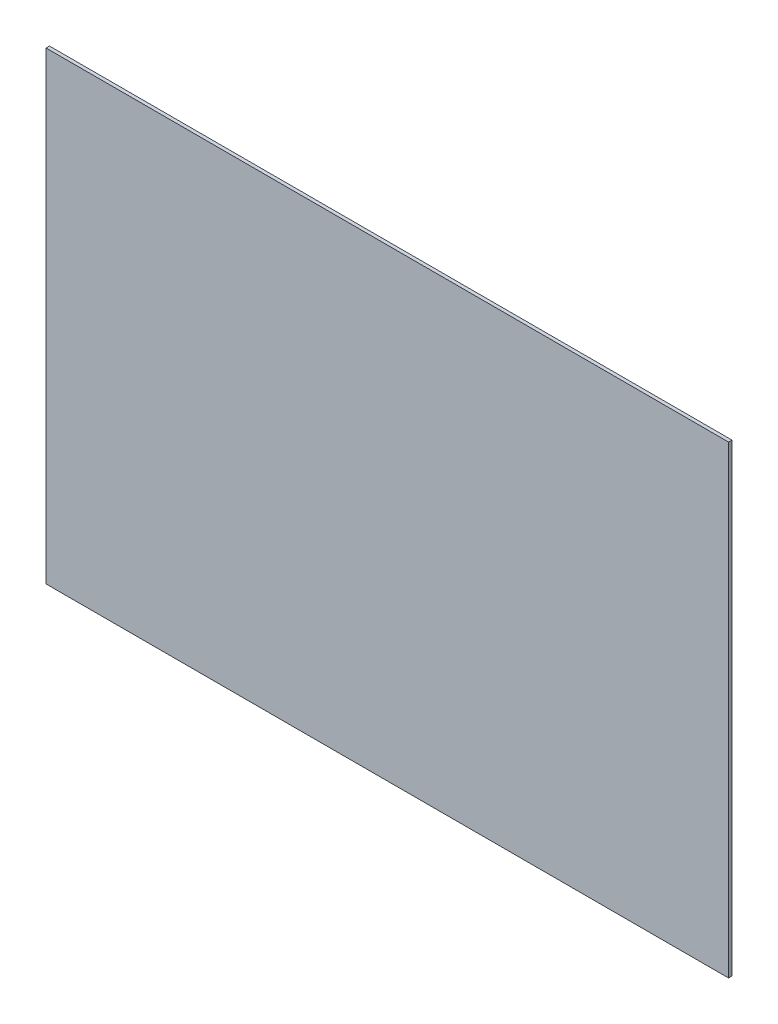
SolidWorks part; units mm, degrees
material "PMMA(有机玻璃)"
ref_plane "前视" through (0, 0, 0) normal (0, 0, 1) x (1, 0, 0)
ref_plane "上视" through (0, 0, 0) normal (0, 1, 0) x (1, 0, 0)
ref_plane "右视" through (0, 0, 0) normal (1, 0, 0) x (0, 0, -1)
sketch "草图1" plane through (0, 0, 0) normal (0, 0, 1) x (1, 0, 0)
  line L1 (-498.5, 339) -> (498.5, 339)
  line L2 (-498.5, 339) -> (-498.5, -339)
  line L3 (-498.5, -339) -> (498.5, -339)
  line L4 (498.5, 339) -> (498.5, -339)
  line L5 (-498.5, 339) -> (498.5, -339) construction
  line L6 (-498.5, -339) -> (498.5, 339) construction
  point P0 (0, 0)
  dimension "D1" = 678
  dimension "D2" = 997
extrude "凸台-拉伸1" add sketch "草图1" along normal blind 5
